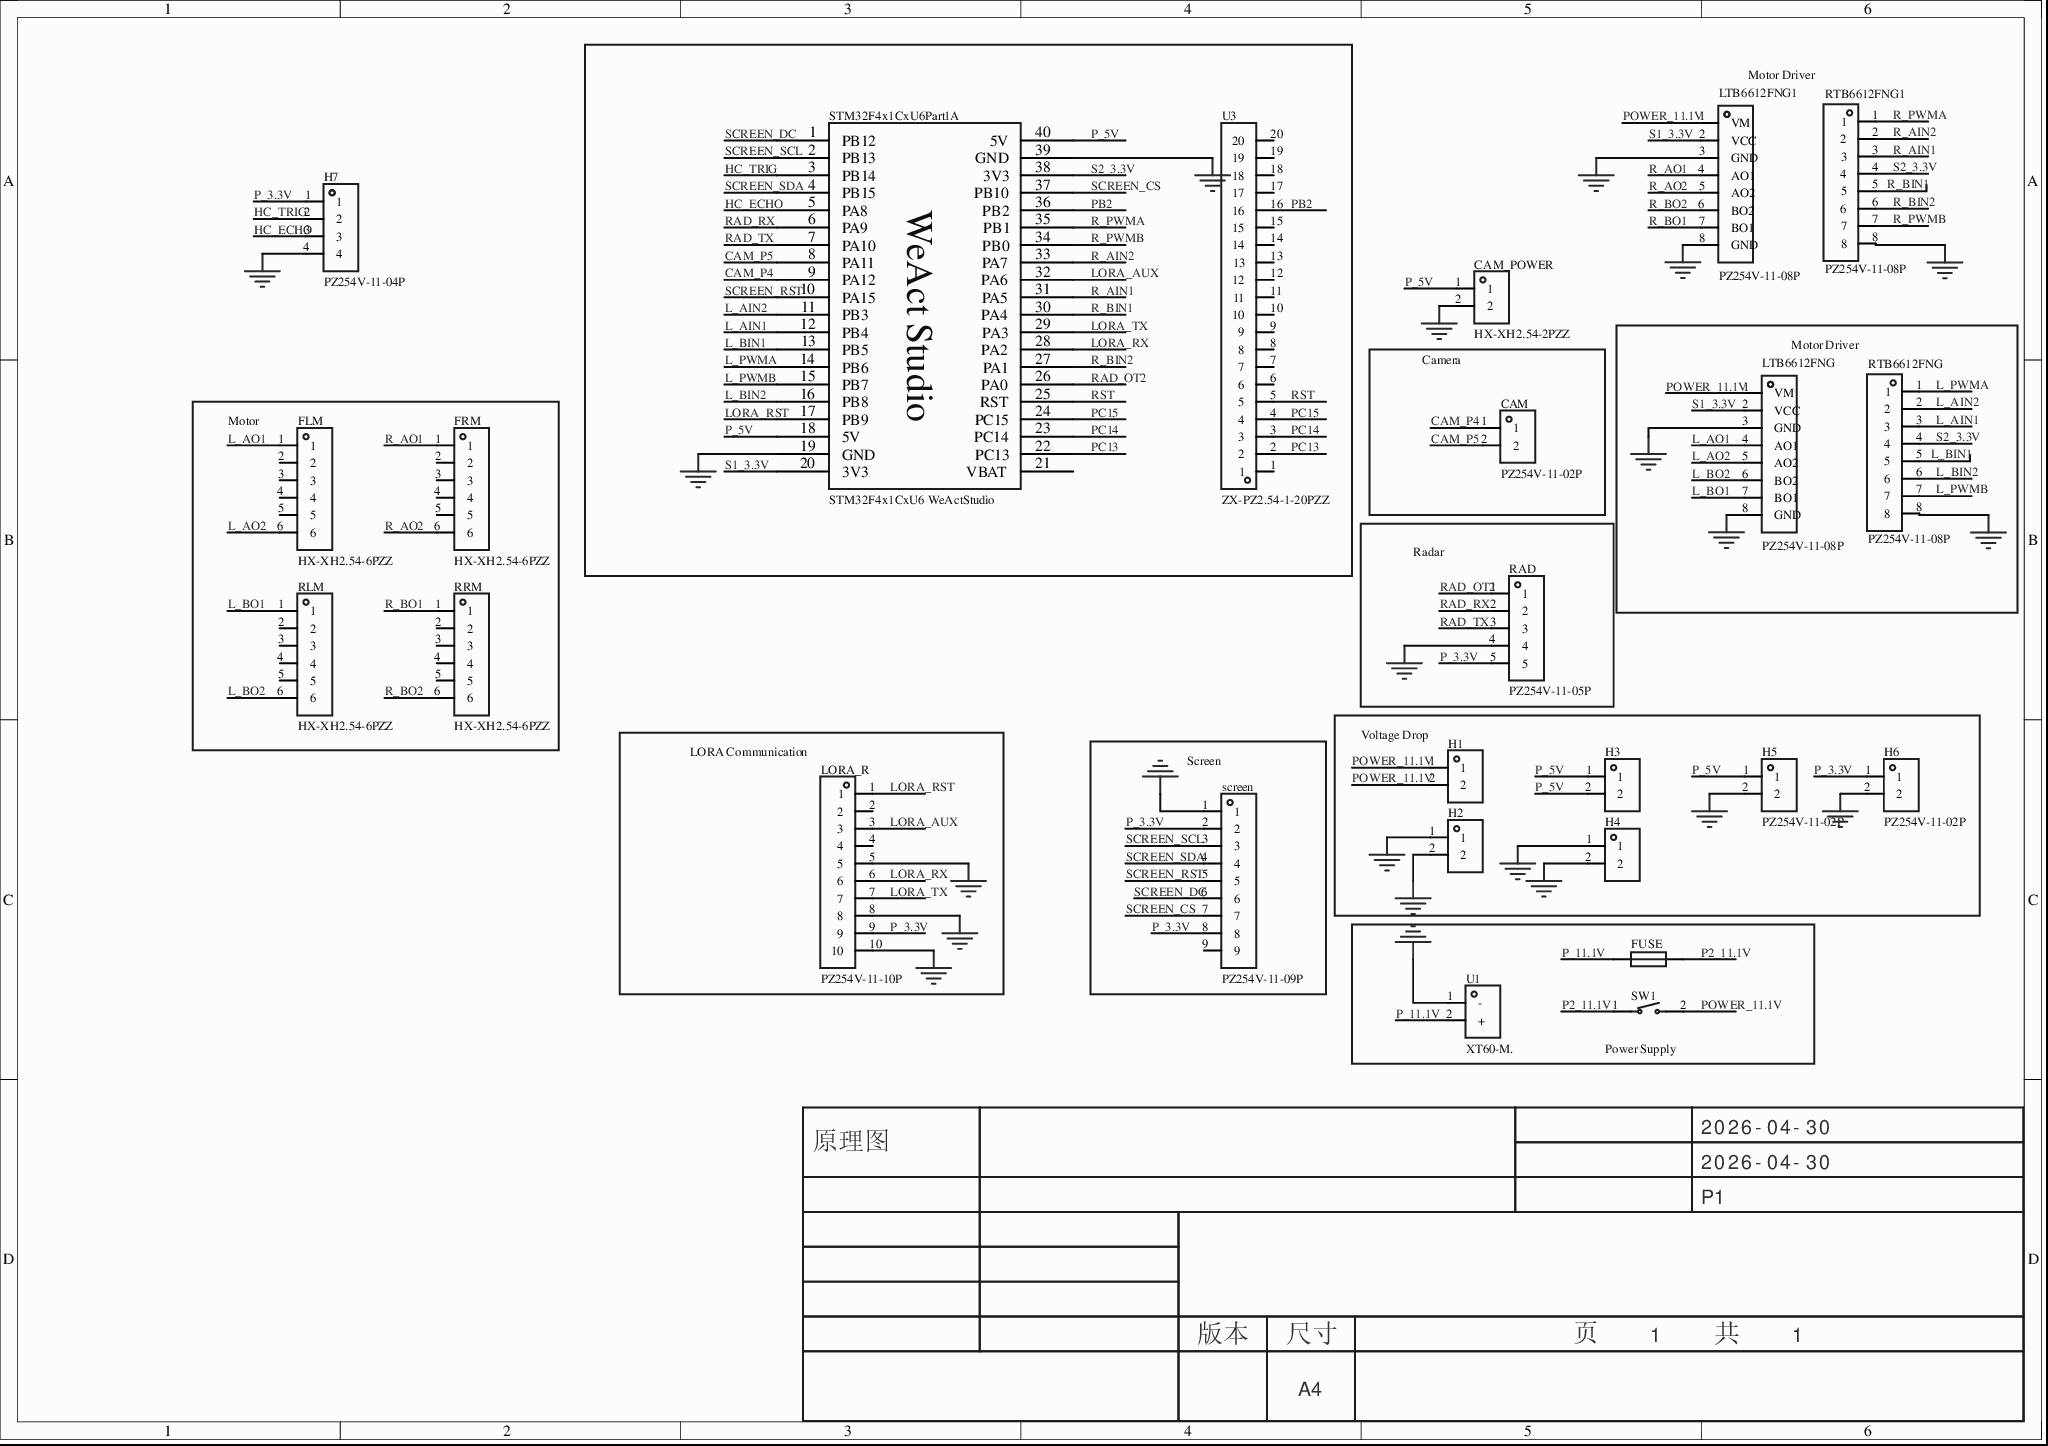
[diagram p0: MISC51978-3.schdoc]
# Altium project MISC51978-2.PrjPcb
1 sheet, 25 parts. Net scope: global (net labels, ports and power ports of the same name join across sheets).
Board file: MISC51978.pcbdoc

## Sheet MISC51978-3.schdoc
size 297 x 209 mm; Version: V1.0; @Project Name: MISC51978; @Update Date: 2026-04-30; @Create Date: 2026-04-30; @Board Name: MISC51978; @Create Time: 14:33:59; @Page Count: 1; @Page No: 1; @Schematic Name: MISC51978; @Update Time: 14:33:59; Size: A4

### Parts
CAM  PZ254V-11-02P  [HDR-TH_2P-P2.54-V-M]
CAM_POWER  HX-XH2.54-2PZZ  [CONN-TH_2P-P2.50_HX-2.54MM-2P-ZZ-MS]
FLM  HX-XH2.54-6PZZ  [CONN-TH_6P-P2.50_BX-XH2.54-6PZZ]
FRM  HX-XH2.54-6PZZ  [CONN-TH_6P-P2.50_BX-XH2.54-6PZZ]
FUSE  (no value)  [F1206]
H1  PZ254V-11-02P  [HDR-TH_2P-P2.54-V-M]  (value not drawn)
H2  PZ254V-11-02P  [HDR-TH_2P-P2.54-V-M]  (value not drawn)
H3  PZ254V-11-02P  [HDR-TH_2P-P2.54-V-M]  (value not drawn)
H4  PZ254V-11-02P  [HDR-TH_2P-P2.54-V-M]  (value not drawn)
H5  PZ254V-11-02P  [HDR-TH_2P-P2.54-V-M]
H6  PZ254V-11-02P  [HDR-TH_2P-P2.54-V-M]
H7  PZ254V-11-04P  [HDR-TH_4P-P2.54-V-M]
LORA_R  PZ254V-11-10P  [HDR-TH_10P-P2.54-V-M]
LTB6612FNG  PZ254V-11-08P  [HDR-TH_8P-P2.54-V-M]
LTB6612FNG1  PZ254V-11-08P  [HDR-TH_8P-P2.54-V-M]
RAD  PZ254V-11-05P  [HDR-TH_5P-P2.54-V-M]
RLM  HX-XH2.54-6PZZ  [CONN-TH_6P-P2.50_BX-XH2.54-6PZZ]
RRM  HX-XH2.54-6PZZ  [CONN-TH_6P-P2.50_BX-XH2.54-6PZZ]
RTB6612FNG  PZ254V-11-08P  [HDR-TH_8P-P2.54-V-M]
RTB6612FNG1  PZ254V-11-08P  [HDR-TH_8P-P2.54-V-M]
screen  PZ254V-11-09P  [HDR-TH_9P-P2.54-V-M]
STM32F4x1CxU6Part1  STM32F4x1CxU6 WeActStudio  [STM32F4x1CxU6 WeActStudio]  (part A of 2)
SW1  HX KCD11-BL  [SW-TH_KCD11-BL]  (value not drawn)
U1  XT60-M.  [CONN-TH_XT60]
U3  ZX-PZ2.54-1-20PZZ  [HDR-TH_20P-P2.54-V-M]

### Blocks framed on the sheet
Camera: CAM
Motor Driver: LTB6612FNG RTB6612FNG
Motor: FLM FRM RLM RRM
Radar: RAD
LORA Communication: LORA_R
Screen: screen
Voltage Drop: H1-H6
Power Supply: FUSE SW1 U1

### Nets
GND: CAM_POWER.2 H2.1 H2.2 H4.1 H4.2 H5.2 H6.2 H7.4 LORA_R.5 LORA_R.8 LORA_R.10 LTB6612FNG.3(GND) LTB6612FNG.8(GND) LTB6612FNG1.3(GND) LTB6612FNG1.8(GND) RAD.4 RTB6612FNG.8 RTB6612FNG1.8 screen.1 STM32F4x1CxU6Part1.19(GND) STM32F4x1CxU6Part1.39(GND) U1.1(-)
CAM_P4: CAM.1 STM32F4x1CxU6Part1.9(PA12)
CAM_P5: CAM.2 STM32F4x1CxU6Part1.8(PA11)
HC_ECHO: H7.3 STM32F4x1CxU6Part1.5(PA8)
HC_TRIG: H7.2 STM32F4x1CxU6Part1.3(PB14)
L_AIN1: RTB6612FNG.3 STM32F4x1CxU6Part1.12(PB4)
L_AIN2: RTB6612FNG.2 STM32F4x1CxU6Part1.11(PB3)
L_AO1: FLM.1 LTB6612FNG.4(AO1)
L_AO2: FLM.6 LTB6612FNG.5(AO2)
L_BIN1: RTB6612FNG.5 STM32F4x1CxU6Part1.13(PB5)
L_BIN2: RTB6612FNG.6 STM32F4x1CxU6Part1.16(PB8)
L_BO1: LTB6612FNG.7(BO1) RLM.1
L_BO2: LTB6612FNG.6(BO2) RLM.6
L_PWMA: RTB6612FNG.1 STM32F4x1CxU6Part1.14(PB6)
L_PWMB: RTB6612FNG.7 STM32F4x1CxU6Part1.15(PB7)
LORA_AUX: LORA_R.3 STM32F4x1CxU6Part1.32(PA6)
LORA_RST: LORA_R.1 STM32F4x1CxU6Part1.17(PB9)
LORA_RX: LORA_R.6 STM32F4x1CxU6Part1.28(PA2)
LORA_TX: LORA_R.7 STM32F4x1CxU6Part1.29(PA3)
P2_11.1V: FUSE.2 SW1.1
P_3.3V: H6.1 H7.1 LORA_R.9 RAD.5 screen.2 screen.8
P_5V: CAM_POWER.1 H3.1 H3.2 H5.1 STM32F4x1CxU6Part1.18(5V) STM32F4x1CxU6Part1.40(5V)
P_11.1V: FUSE.1 U1.2(+)
PB2: STM32F4x1CxU6Part1.36(PB2) U3.16
PC13: STM32F4x1CxU6Part1.22(PC13) U3.2
PC14: STM32F4x1CxU6Part1.23(PC14) U3.3
PC15: STM32F4x1CxU6Part1.24(PC15) U3.4
POWER_11.1V: H1.1 H1.2 LTB6612FNG.1(VM) LTB6612FNG1.1(VM) SW1.2
R_AIN1: RTB6612FNG1.3 STM32F4x1CxU6Part1.31(PA5)
R_AIN2: RTB6612FNG1.2 STM32F4x1CxU6Part1.33(PA7)
R_AO1: FRM.1 LTB6612FNG1.4(AO1)
R_AO2: FRM.6 LTB6612FNG1.5(AO2)
R_BIN1: RTB6612FNG1.5 STM32F4x1CxU6Part1.30(PA4)
R_BIN2: RTB6612FNG1.6 STM32F4x1CxU6Part1.27(PA1)
R_BO1: LTB6612FNG1.7(BO1) RRM.1
R_BO2: LTB6612FNG1.6(BO2) RRM.6
R_PWMA: RTB6612FNG1.1 STM32F4x1CxU6Part1.35(PB1)
R_PWMB: RTB6612FNG1.7 STM32F4x1CxU6Part1.34(PB0)
RAD_OT2: RAD.1 STM32F4x1CxU6Part1.26(PA0)
RAD_RX: RAD.2 STM32F4x1CxU6Part1.6(PA9)
RAD_TX: RAD.3 STM32F4x1CxU6Part1.7(PA10)
RST: STM32F4x1CxU6Part1.25(RST) U3.5
S1_3.3V: LTB6612FNG.2(VCC) LTB6612FNG1.2(VCC) STM32F4x1CxU6Part1.20(3V3)
S2_3.3V: RTB6612FNG.4 RTB6612FNG1.4 STM32F4x1CxU6Part1.38(3V3)
SCREEN_CS: screen.7 STM32F4x1CxU6Part1.37(PB10)
SCREEN_DC: screen.6 STM32F4x1CxU6Part1.1(PB12)
SCREEN_RST: screen.5 STM32F4x1CxU6Part1.10(PA15)
SCREEN_SCL: screen.3 STM32F4x1CxU6Part1.2(PB13)
SCREEN_SDA: screen.4 STM32F4x1CxU6Part1.4(PB15)

Not connected (* = marked no-connect by the designer): FLM 2* 3* 4* 5*; FRM 2* 3* 4* 5*; LORA_R 2* 4*; RLM 2* 3* 4* 5*; RRM 2* 3* 4* 5*; screen 9*; STM32F4x1CxU6Part1 21(VBAT)*; U3 1* 6* 7* 8* 9* 10* 11* 12* 13* 14* 15* 17* 18* 19* 20*

### Notes on the sheet
- Motor Driver
- 2026-04-30
- 原理图
- P1
- 版本
- 尺寸
- A4
- 页    1    共    1

### Library data of the parts
CAM H1-H6 = PZ254V-11-02P: 插针结构:1x2P;间距:2.54mm;行距:-;圆针/方针:方针;安装方式:直插;排数:单排;总PIN位数:2P;额定电流:3A;额定电压:250V;配合针长度:6mm;塑高:2.5mm;端接针长度:3mm;触头材质:黄铜;触头镀层:-;工作温度:-40℃~+105℃;颜色:黑色;; Manufacturer: XFCN(兴飞); 3D Model: e35305ec3aa84b66b849f914b715e73f0819f05c4eef4c71ace90d822a990e87; 3D Model Transform: 200,100,0,0,0,0,0,0,-118.11; Pin Structure: 1x2P; Pitch: 2.54mm; Circluar Pins/Square Pins: 方针; Current Rating: 3A; Voltage Rating (Max): 250V; AddInBom: yes; ModelName: HDR2.54-M-LI-1X2P; Symbol: PZ254V-11-02P; Device: PZ254V-11-02P; LCSC Part Name: 1x2P 间距:2.54mm 方针 直插; Supplier Part: C492401; Manufacturer Part: PZ254V-11-02P; Supplier Footprint: 插件,P=2.54mm; JLCPCB Part Class: Extended Part; Datasheet: https://item.szlcsc.com/datasheet/PZ254V-11-02P/502957.html; Supplier: LCSC; Row Spacing: -; Mounting Type: 直插; Number of Rows: 单排; Number of Pins: 2P; Length of Mating Pin: 6mm; Insulation Height: 2.5mm; Length of End Connection Pin: 3mm; Contact Material: 黄铜; Contact Plating: -; Operating Temperature: -40℃~+105℃; Color: 黑色; ConvertToPcb: yes; FootprintName: HDR-TH_2P-P2.54-V-M
CAM_POWER = HX-XH2.54-2PZZ: 插针结构:1x2P;间距:2.54mm;安装方式:直插;参考系列:XH;总PIN数:2P;排数:1;每排PIN数:2;行距:-;额定电流:3A;触头材质:黄铜;触头镀层:锡;工作温度:-25℃~+85℃;; Manufacturer: hanxia(韩下); AddInBom: yes; ModelId: 1cafe43f43c04794b29c478db770ea2f0819f05c4eef4c71ace90d822a990e87; ModelTransform: 295.275,228.7397,0,0,0,0,0,-19.685,-137.795; Pins Structure: 1x2P; Pitch: 2.54mm; Reference Series: XH; Number of PINs Per Row: 2; Current Rating: 3A; Voltage Rating: 250V; Plastic Material: PA66; Flame Retardant Rating: UL94V-0; Symbol: HX-XH2.54-2PZZ; Device: HX-XH2.54-2PZZ; LCSC Part Name: 1x2P 间距:2.5mm 直插 系列:XH; SupplierPart: C42391660; ManufacturerPart: HX-XH2.54-2PZZ; Supplier Footprint: 插件,P=2.5mm; JLCPCB Part Class: Extended Part; Datasheet: https://item.szlcsc.com/datasheet/HX-XH2.54-2PZZ/44326932.html; Supplier: LCSC; ConvertToPcb: yes; FootprintName: CONN-TH_2P-P2.50_HX-2.54MM-2P-ZZ-MS; ModelName: CONN-TH_2P-P2.50_HX-2.54MM-2P-ZZ-MS; Mounting Type: 直插; Number of Pins: 2P; Number of Rows: 1; Row Spacing: -; Contact Material: 黄铜; Contact Plating: 锡; Operating Temperature: -25℃~+85℃; Color: 白色
FLM FRM RLM RRM = HX-XH2.54-6PZZ: 插针结构:1x6P;间距:2.54mm;安装方式:直插;参考系列:XH;总PIN数:6P;排数:1;每排PIN数:6;行距:-;额定电流:3A;触头材质:黄铜;触头镀层:锡;工作温度:-25℃~+85℃;; Manufacturer: hanxia(韩下); AddInBom: yes; ModelId: 339169ddee9a410aa0e9978eac1327870819f05c4eef4c71ace90d822a990e87; ModelTransform: 688.975,232.6767,0,0,0,0,-0.005,18.898,-133.858; Pins Structure: 1x6P; Pitch: 2.54mm; Reference Series: XH; Number of PINs Per Row: 6; Current Rating: 3A; Voltage Rating: 250V; Plastic Material: PA66; Flame Retardant Rating: UL94V-0; Symbol: HX-XH2.54-6PZZ; Device: HX-XH2.54-6PZZ; LCSC Part Name: 1x6P 间距:2.54mm 直插 系列:XH; SupplierPart: C42391664; ManufacturerPart: HX-XH2.54-6PZZ; Supplier Footprint: 插件,P=2.5mm; JLCPCB Part Class: Extended Part; Datasheet: https://item.szlcsc.com/datasheet/HX-XH2.54-6PZZ/44326936.html; Supplier: LCSC; ConvertToPcb: yes; FootprintName: CONN-TH_6P-P2.50_BX-XH2.54-6PZZ; ModelName: CONN-TH_6P-P2.50_BX-XH2.54-6PZZ; Mounting Type: 直插; Number of Pins: 6P; Number of Rows: 1; Row Spacing: -; Contact Material: 黄铜; Contact Plating: 锡; Operating Temperature: -25℃~+85℃; Color: 白色
FUSE = QF1206F3A00T: 类型:贴片式保险丝;额定电流:3A;额定电压:32V;分断能力:50A@32VDC;; Manufacturer: AEM; AddInBom: yes; ModelId: f1628daad26847a79b887277a2bc85410819f05c4eef4c71ace90d822a990e87; ModelName: F1206_L3.2-W1.7-H0.6; ModelTransform: 125.984,66.929,0,0,0,0,0,0,0; Current Rating: 3A; Voltage Rating (DC): 32V; Melting I2t: 0.22; Symbol: QF1206F3A00T; Device: QF1206F3A00T; LCSC Part Name: 32V 3A; SupplierPart: C2992307; Supplier Footprint: 1206; JLCPCB Part Class: Extended Part; Datasheet: https://item.szlcsc.com/datasheet/QF1206F3A00T/3456635.html; Supplier: LCSC; ConvertToPcb: yes; FootprintName: F1206; Type: 贴片式保险丝; Interrupt Rating: 50A@32VDC; Length: 3.2mm; Width: 1.6mm; Height: 0.85mm
H7 = PZ254V-11-04P: 插针结构:1x4P;间距:2.54mm;行距:-;圆针/方针:方针;安装方式:直插;排数:单排;总PIN位数:4P;额定电流:3A;额定电压:250V;配合针长度:6mm;塑高:2.5mm;端接针长度:3mm;触头材质:-;工作温度:-40℃~+105℃;颜色:黑色;; Manufacturer: XFCN(兴飞); Symbol: PZ254V-11-04P_C2691448; 3D Model: 112f4d05e8d64e99ab9a333894bea4f90819f05c4eef4c71ace90d822a990e87; 3D Model Transform: 399.999,104.7242,0,0,0,0,0,0,-118.11; Pin Structure: 1x4P; Pitch: 2.54mm; Circluar Pins/Square Pins: 方针; Current Rating: 3A; Voltage Rating (Max): 250V; AddInBom: yes; ModelName: HDR-TH_4P-P2.54-M-LI-1X4P; Device: PZ254V-11-04P; LCSC Part Name: 1x4P 间距:2.54mm 方针 直插; Supplier Part: C2691448; Manufacturer Part: PZ254V-11-04P; Supplier Footprint: 插件,P=2.54mm; JLCPCB Part Class: Extended Part; Datasheet: https://item.szlcsc.com/datasheet/PZ254V-11-04P/2801085.html; Supplier: LCSC; Row Spacing: -; Mounting Type: 直插; Number of Rows: 单排; Number of Pins: 4P; Length of Mating Pin: 6mm; Insulation Height: 2.5mm; Length of End Connection Pin: 3mm; Contact Material: -; Operating Temperature: -40℃~+105℃; Color: 黑色; ConvertToPcb: yes; FootprintName: HDR-TH_4P-P2.54-V-M
LORA_R = PZ254V-11-10P: 插针结构:1x10P;间距:2.54mm;行距:-;圆针/方针:方针;安装方式:直插;排数:单排;总PIN位数:10P;额定电流:3A;额定电压:250V;配合针长度:6mm;塑高:2.5mm;端接针长度:3mm;触头材质:黄铜;触头镀层:-;工作温度:-40℃~+105℃;颜色:黑色;; Manufacturer: XFCN(兴飞); AddInBom: yes; ModelId: 10f3d1cea59e4bb4ba116af9f09c2b9b0819f05c4eef4c71ace90d822a990e87; ModelName: HDR2.54-M-LI-1X10P; ModelTransform: 999.99796,100,0,0,0,0,0,0,-118.11; Pin Structure: 1x10P; Pitch: 2.54mm; Circluar Pins/Square Pins: 方针; Current Rating: 3A; Voltage Rating (Max): 250V; Symbol: PZ254V-11-10P; Device: PZ254V-11-10P; LCSC Part Name: 1x10P 间距:2.54mm 方针 直插; SupplierPart: C492409; ManufacturerPart: PZ254V-11-10P; Supplier Footprint: 插件,P=2.54mm; JLCPCB Part Class: Extended Part; Datasheet: https://item.szlcsc.com/datasheet/PZ254V-11-10P/502965.html; Supplier: LCSC; ConvertToPcb: yes; FootprintName: HDR-TH_10P-P2.54-V-M; Row Spacing: -; Mounting Type: 直插; Number of Rows: 单排; Number of Pins: 10P; Length of Mating Pin: 6mm; Insulation Height: 2.5mm; Length of End Connection Pin: 3mm; Contact Material: 黄铜; Contact Plating: -; Operating Temperature: -40℃~+105℃; Color: 黑色
LTB6612FNG LTB6612FNG1 = PZ254V-11-08P: 插针结构:1x8P;间距:2.54mm;行距:-;圆针/方针:方针;安装方式:直插;排数:单排;总PIN位数:8P;额定电流:3A;额定电压:250V;配合针长度:6mm;塑高:2.5mm;端接针长度:3mm;触头材质:黄铜;触头镀层:-;工作温度:-40℃~+105℃;颜色:黑色;; Manufacturer: XFCN(兴飞); Symbol: PZ254V-11-08P_2; 3D Model: f5b96e27511e49e38545e53df23202020819f05c4eef4c71ace90d822a990e87; 3D Model Transform: 807.87244,98.425,0,0,0,0,0,0,-118.11; Pin Structure: 1x8P; Pitch: 2.54mm; Circluar Pins/Square Pins: 方针; Current Rating: 3A; Voltage Rating (Max): 250V; AddInBom: yes; Device: PZ254V-11-08P; LCSC Part Name: 1x8P 间距:2.54mm 方针 直插; Supplier Part: C492407; Manufacturer Part: PZ254V-11-08P; Supplier Footprint: 插件,P=2.54mm; JLCPCB Part Class: Extended Part; Datasheet: https://item.szlcsc.com/datasheet/PZ254V-11-08P/502963.html; Supplier: LCSC; Row Spacing: -; Mounting Type: 直插; Number of Rows: 单排; Number of Pins: 8P; Length of Mating Pin: 6mm; Insulation Height: 2.5mm; Length of End Connection Pin: 3mm; Contact Material: 黄铜; Contact Plating: -; Operating Temperature: -40℃~+105℃; Color: 黑色; ConvertToPcb: yes; FootprintName: HDR-TH_8P-P2.54-V-M; ModelName: HDR-TH_8P-P2.54-V-M
RAD = PZ254V-11-05P: 插针结构:1x5P;间距:2.54mm;行距:-;圆针/方针:方针;安装方式:直插;排数:单排;总PIN位数:5P;额定电流:3A;额定电压:250V;配合针长度:6mm;塑高:2.5mm;端接针长度:3mm;触头材质:黄铜;触头镀层:-;工作温度:-40℃~+105℃;颜色:黑色;; Manufacturer: XFCN(兴飞); AddInBom: yes; ModelId: 47d466e4a34f4fc5bc626cf773a24dd50819f05c4eef4c71ace90d822a990e87; ModelName: HDR-TH_5P-P2.54-M-LI-1X5P; ModelTransform: 499.999,100,0,0,0,0,0,0,-118.11; Pin Structure: 1x5P; Pitch: 2.54mm; Circluar Pins/Square Pins: 方针; Current Rating: 3A; Voltage Rating (Max): 250V; Symbol: PZ254V-11-05P; Device: PZ254V-11-05P; LCSC Part Name: 1x5P 间距:2.54mm 方针 直插; SupplierPart: C492404; ManufacturerPart: PZ254V-11-05P; Supplier Footprint: 插件,P=2.54mm; JLCPCB Part Class: Extended Part; Datasheet: https://item.szlcsc.com/datasheet/PZ254V-11-05P/502960.html; Supplier: LCSC; ConvertToPcb: yes; FootprintName: HDR-TH_5P-P2.54-V-M; Row Spacing: -; Mounting Type: 直插; Number of Rows: 单排; Number of Pins: 5P; Length of Mating Pin: 6mm; Insulation Height: 2.5mm; Length of End Connection Pin: 3mm; Contact Material: 黄铜; Contact Plating: -; Operating Temperature: -40℃~+105℃; Color: 黑色
RTB6612FNG RTB6612FNG1 = PZ254V-11-08P: 插针结构:1x8P;间距:2.54mm;行距:-;圆针/方针:方针;安装方式:直插;排数:单排;总PIN位数:8P;额定电流:3A;额定电压:250V;配合针长度:6mm;塑高:2.5mm;端接针长度:3mm;触头材质:黄铜;触头镀层:-;工作温度:-40℃~+105℃;颜色:黑色;; Manufacturer: XFCN(兴飞); 3D Model: f5b96e27511e49e38545e53df23202020819f05c4eef4c71ace90d822a990e87; 3D Model Transform: 807.87244,98.425,0,0,0,0,0,0,-118.11; Pin Structure: 1x8P; Pitch: 2.54mm; Circluar Pins/Square Pins: 方针; Current Rating: 3A; Voltage Rating (Max): 250V; AddInBom: yes; Symbol: PZ254V-11-08P; Device: PZ254V-11-08P; LCSC Part Name: 1x8P 间距:2.54mm 方针 直插; Supplier Part: C492407; Manufacturer Part: PZ254V-11-08P; Supplier Footprint: 插件,P=2.54mm; JLCPCB Part Class: Extended Part; Datasheet: https://item.szlcsc.com/datasheet/PZ254V-11-08P/502963.html; Supplier: LCSC; Row Spacing: -; Mounting Type: 直插; Number of Rows: 单排; Number of Pins: 8P; Length of Mating Pin: 6mm; Insulation Height: 2.5mm; Length of End Connection Pin: 3mm; Contact Material: 黄铜; Contact Plating: -; Operating Temperature: -40℃~+105℃; Color: 黑色; ConvertToPcb: yes; FootprintName: HDR-TH_8P-P2.54-V-M; ModelName: HDR-TH_8P-P2.54-V-M
screen = PZ254V-11-09P: 插针结构:1x9P;间距:2.54mm;行距:-;圆针/方针:方针;安装方式:直插;排数:单排;总PIN位数:9P;额定电流:3A;额定电压:250V;配合针长度:6mm;塑高:2.5mm;端接针长度:3mm;触头材质:黄铜;触头镀层:-;工作温度:-40℃~+105℃;颜色:黑色;; Manufacturer: XFCN(兴飞); AddInBom: yes; ModelId: b5c1e988b3bb4503807579736b357ad00819f05c4eef4c71ace90d822a990e87; ModelName: HDR-TH_9P-P2.54-M-LI-1X9P; ModelTransform: 890.15562,98.425,0,0,0,0,0,0,-118.11; Pin Structure: 1x9P; Pitch: 2.54mm; Circluar Pins/Square Pins: 方针; Current Rating: 3A; Voltage Rating (Max): 250V; Symbol: PZ254V-11-09P; Device: PZ254V-11-09P; LCSC Part Name: 1x9P 间距:2.54mm 方针 直插; SupplierPart: C492408; ManufacturerPart: PZ254V-11-09P; Supplier Footprint: 插件,P=2.54mm; JLCPCB Part Class: Extended Part; Datasheet: https://item.szlcsc.com/datasheet/PZ254V-11-09P/502964.html; Supplier: LCSC; ConvertToPcb: yes; FootprintName: HDR-TH_9P-P2.54-V-M; Row Spacing: -; Mounting Type: 直插; Number of Rows: 单排; Number of Pins: 9P; Length of Mating Pin: 6mm; Insulation Height: 2.5mm; Length of End Connection Pin: 3mm; Contact Material: 黄铜; Contact Plating: -; Operating Temperature: -40℃~+105℃; Color: 黑色
STM32F4x1CxU6Part1 = STM32F4x1CxU6 WeActStudio: STM32F4x1CxU6; Relevance: []; componentDisplayMode: -1; AddInBom: yes; Symbol: STM32F4x1CxU6 WeActStudio; Device: STM32F4x1CxU6 WeActStudio; ComponentLink1Description: WeAct Studio; ComponentLink2Description: MiniF4-STM32F4x1 Github; ComponentLink3Description: MiniF4-STM32F4x1 Gitee; FootprintName: STM32F4x1CxU6 WeActStudio; OriginFootprint: STM32F4x1CxU6 WeActStudio
SW1 = HX KCD11-BL: 带灯:无;引脚样式:焊片;额定电流:3A;额定电压(AC):250V;电路结构:单刀单掷;工作寿命:1万次;; Manufacturer: hanxia(韩下); AddInBom: yes; ModelId: 0d182dc3e1174bea8b4d981fec7704a50819f05c4eef4c71ace90d822a990e87; ModelTransform: 893.699,335.0387,0,90,0,0,0,-343.897,-137.795; With Lamp: 无; Actuator Color: 黑色; Current Rating: 3A; Voltage Rating (AC): 250V; Circuit: 单刀单掷; Life: 1万次; Symbol: HX KCD11-BL; Device: HX KCD11-BL; LCSC Part Name: 8.5*13.5mm 两脚两档跷板开关 弯脚黑色; SupplierPart: C6917329; ManufacturerPart: HX KCD11-BL; Supplier Footprint: 插件; JLCPCB Part Class: Extended Part; Datasheet: https://item.szlcsc.com/datasheet/HX%2520KCD11-BL/7881941.html; Supplier: LCSC; ConvertToPcb: yes; FootprintName: SW-TH_KCD11-BL; ModelName: SW-TH_KCD11-BL; Termination Style: 焊片
U1 = XT60-M.: 模型锂电连接器 XT60-M; Manufacturer: AMASS(艾迈斯); Symbol: XT60; AddInBom: yes; ModelId: 185081e4ebbe4eaea4bbf508888b62e20819f05c4eef4c71ace90d822a990e87; ModelTransform: 610.235,319.291,0,0,0,0,0,0,-196.85; Connector type: 香蕉头; interface form: 公头; Device: XT60-M.; LCSC Part Name: AMASS(艾迈斯)XT60模型插头出线焊接式  2P 镀金 公头XT60-M.G.Y; SupplierPart: C98733; ManufacturerPart: XT60-M.; Supplier Footprint: -; JLCPCB Part Class: Extended Part; Datasheet: https://item.szlcsc.com/datasheet/XT60-M./99943.html; Supplier: LCSC; ConvertToPcb: yes; FootprintName: CONN-TH_XT60; ModelName: CONN-TH_XT60; colour: 黄色; Size/Specification: 3.5mm
U3 = ZX-PZ2.54-1-20PZZ: 插针结构:1x20P;间距:2.54mm;行距:-;圆针/方针:方针;安装方式:直插;排数:单排;总PIN位数:20P;额定电流:3A;额定电压:-;配合针长度:6mm;塑高:2.5mm;端接针长度:3mm;触头材质:黄铜;触头镀层:金;工作温度:-40℃~+105℃;颜色:黑色;; Manufacturer: Megastar(兆星); AddInBom: yes; ModelId: f68709be121d406db68b06f32a5953890819f05c4eef4c71ace90d822a990e87; ModelName: HDR-M-2.54_1x20; ModelTransform: 1999.996,100,0,0,0,0,0,0,-118.11; Pin Structure: 1x20P; Pitch: 2.54mm; Circluar Pins/Square Pins: 方针; Current Rating: 3A; Symbol: ZX-PZ2.54-1-20PZZ; Device: ZX-PZ2.54-1-20PZZ; LCSC Part Name: 1x20P 间距:2.54mm 方针 直插; SupplierPart: C7501271; ManufacturerPart: ZX-PZ2.54-1-20PZZ; Supplier Footprint: 插件,P=2.54mm; JLCPCB Part Class: Extended Part; Datasheet: https://item.szlcsc.com/datasheet/ZX-PZ2.54-1-20PZZ/8582484.html; Supplier: LCSC; ConvertToPcb: yes; FootprintName: HDR-TH_20P-P2.54-V-M; Row Spacing: -; Mounting Type: 直插; Number of Rows: 单排; Number of Pins: 20P; Voltage Rating (Max): -; Length of Mating Pin: 6mm; Insulation Height: 2.5mm; Length of End Connection Pin: 3mm; Contact Material: 黄铜; Contact Plating: 金; Operating Temperature: -40℃~+105℃; Color: 黑色